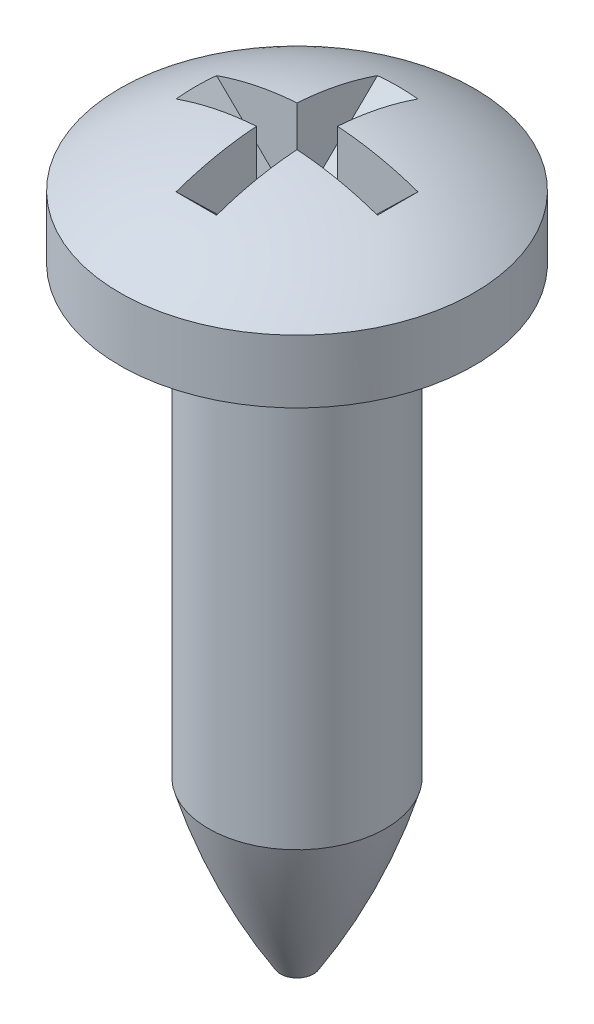
from build123d import *

# Parameters (mm, degrees)
SKETCH2_R           = 1.75
BOSS_EXTRUDE1_DEPTH = 8.8
CUT_EXTRUDE1_DEPTH  = 0.4
CIRPATTERN1_COUNT   = 4


with BuildPart() as part:
    # Sketch1 → Revolve2 (revolve)
    with BuildSketch(Plane.XY, mode=Mode.PRIVATE) as revolve2_sk:
        with BuildLine():
            Line((0, 3.8596837944664038), (3.5000000000000013, 3.8596837944664038))
            Line((3.5000000000000013, 3.8596837944664038), (3.5000000000000013, 5.104743083003953))
            ThreePointArc((3.5000000000000013, 5.104743083003953), (1.8384255445316686, 5.9427548013385545), (8.7e-16, 6.231345910599472))
            Line((8.7e-16, 6.231345910599472), (0, 3.8596837944664038))
        make_face()
    revolve(revolve2_sk.sketch.rotate(Axis((0, 9.918972332015809, 0), (2.4e-16, -1, 0)), 180), axis=Axis((0, 9.918972332015809, 0), (2.4e-16, -1, 0)))

    # Sketch2 → Boss-Extrude1 (add)
    with BuildSketch(Plane.XZ.offset(-3.8596837944664033)):
        Circle(SKETCH2_R)
    extrude(amount=BOSS_EXTRUDE1_DEPTH)

    # Sketch3 → Revolve3 (revolve)
    with BuildSketch(Plane.XY, mode=Mode.PRIVATE) as revolve3_sk:
        with BuildLine():
            Line((-0.3268895580285352, -8.140316205533598), (0, -8.140316205533598))
            Line((0, -8.140316205533598), (-3.69e-15, -4.940316205533597))
            Line((-3.69e-15, -4.940316205533597), (-1.7500000000000084, -4.940316205533597))
            ThreePointArc((-1.7500000000000084, -4.940316205533597), (-1.148404721070234, -6.5892178123268526), (-0.3268895580285352, -8.140316205533598))
        make_face()
    revolve(revolve3_sk.sketch.rotate(Axis((0, 0, 0), (0, -1, 0)), 180), axis=Axis((0, 0, 0), (0, -1, 0)))

    # Sketch8 → Cut-Extrude1 (cut, symmetric)
    with BuildSketch(Plane.XY):
        with BuildLine():
            Line((-2, 5.888200160091848), (-0.3999999999999996, 4.331345910599471))
            Line((-0.3999999999999996, 4.331345910599471), (0.40000000000000047, 4.33134591059947))
            Line((0.40000000000000047, 4.33134591059947), (2, 5.8882001600918485))
            ThreePointArc((2, 5.8882001600918485), (3.4e-16, 6.231345910599467), (-2, 5.888200160091848))
        make_face()
    cut_extrude1 = extrude(amount=CUT_EXTRUDE1_DEPTH, both=True, mode=Mode.SUBTRACT)

    # CirPattern1: Cut-Extrude1 ×4 about axis
    cirpattern1_axis = Axis((3.1e-16, 0, 3.1e-16), (0, 1, 0))
    for i in range(1, CIRPATTERN1_COUNT):
        add(cut_extrude1.rotate(cirpattern1_axis, i * 360 / CIRPATTERN1_COUNT), mode=Mode.SUBTRACT)


solid = part.part
